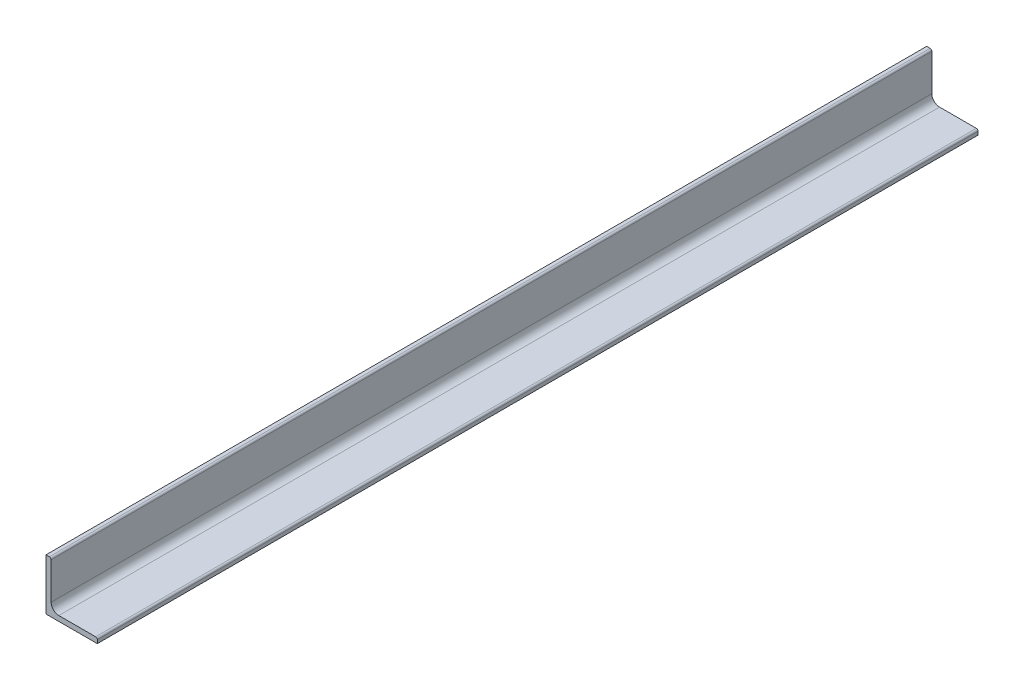
from build123d import *

# Parameters (mm, degrees)
BOSS_EXTRUDE1_DEPTH = 257.5


with BuildPart() as part:
    # Sketch1 → Boss-Extrude1 (new, symmetric)
    with BuildSketch(Plane.XY):
        with BuildLine():
            Line((0, 0), (0, 30))
            Line((0, 30), (2, 30))
            ThreePointArc((2, 30), (2.707106781, 29.707106781), (3, 29))
            Line((3, 29), (3, 7.5))
            ThreePointArc((3, 7.5), (4.318019485, 4.318019485), (7.5, 3))
            Line((7.5, 3), (29, 3))
            ThreePointArc((29, 3), (29.707106781, 2.707106781), (30, 2))
            Line((30, 2), (30, 0))
            Line((30, 0), (0, 0))
        make_face()
    extrude(amount=BOSS_EXTRUDE1_DEPTH, both=True)


solid = part.part
